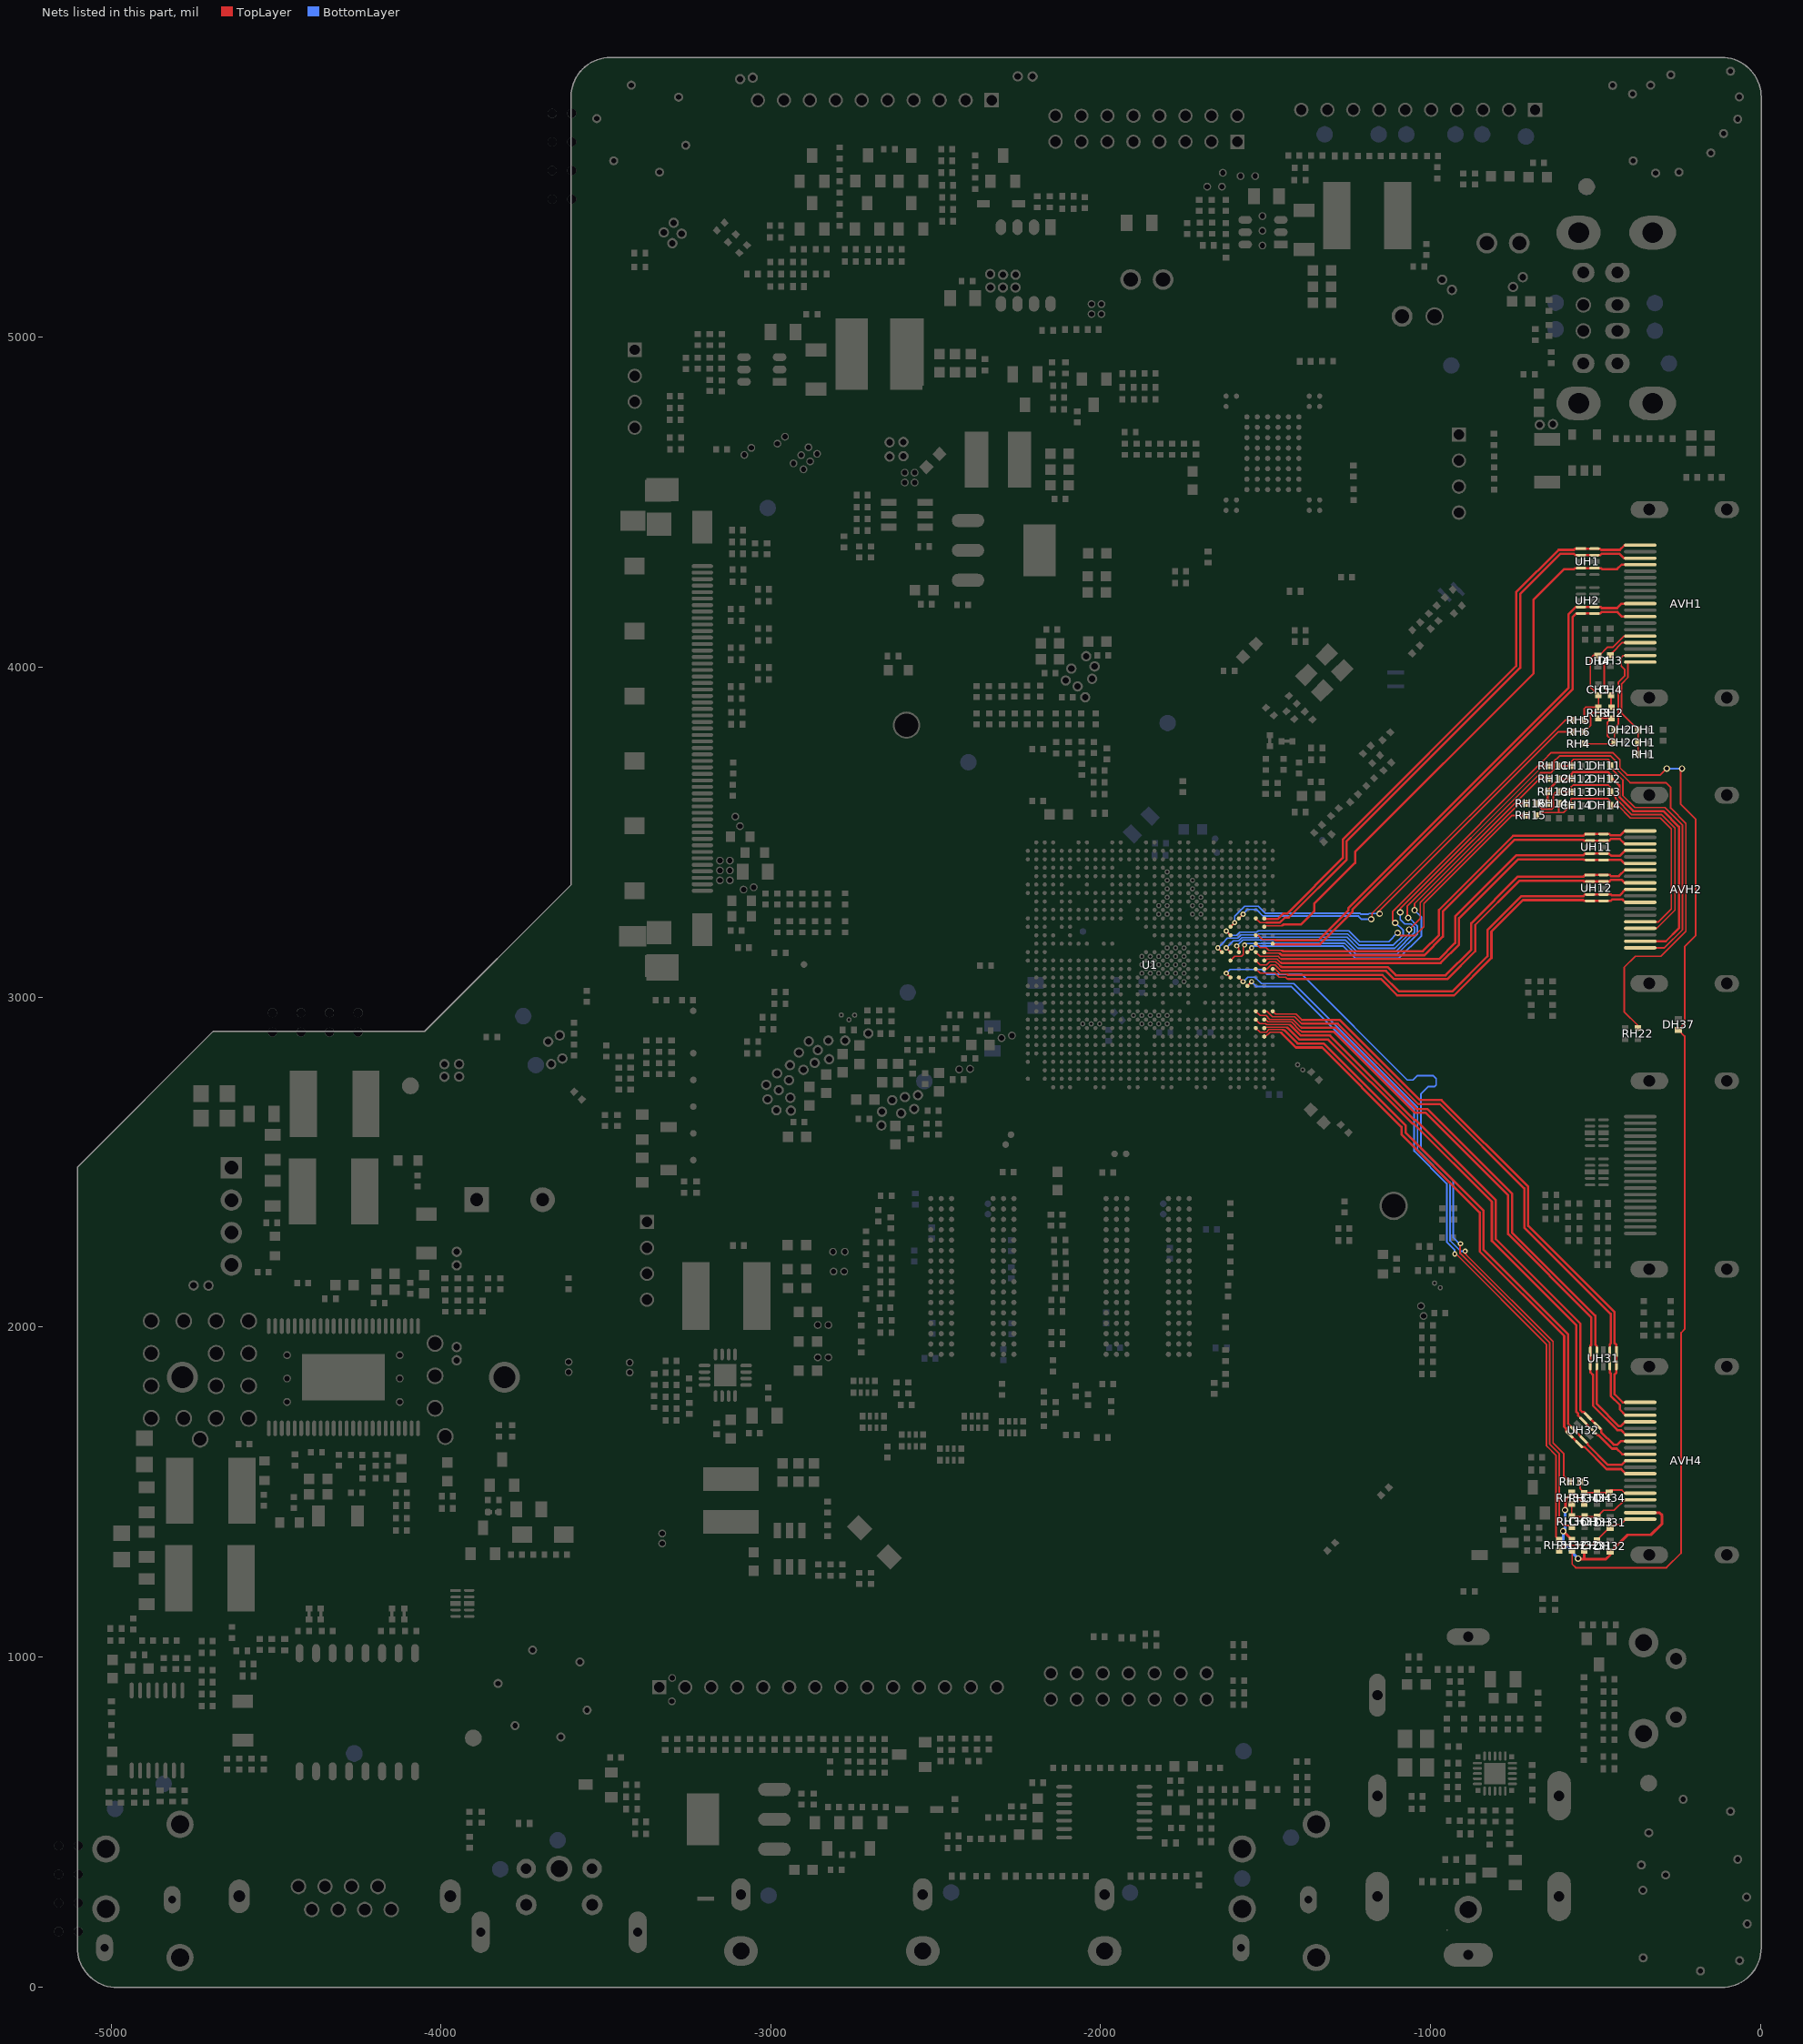
[diagram p0: the nets of this part, all layers, seen from the top]
# Altium PCB MISC86290.PcbDoc (part 22 of 31)
Units mil, origin at the board's own origin, x right, y up, seen from the top; angles counter-clockwise.
Board outline 5104.71 x 5851.49 mil, 2 copper layers (TopLayer, BottomLayer), stack 61.855 mil thick; 1026 components, 667 nets, 4280 pads, 2294 vias.

## Via types
v1: diameter 19.68, hole 11.81, TopLayer to BottomLayer, tented both sides, 1189 vias
v2: diameter 19.68/19.68 (per signal layer), hole 11.81, TopLayer to BottomLayer, tented both sides, 366 vias
v3: diameter 15.75, hole 7.87, TopLayer to BottomLayer, tented both sides, 348 vias
v4: diameter 23.62, hole 15.75, TopLayer to BottomLayer, tented both sides, 309 vias
v5: diameter 15.75/15.75 (per signal layer), hole 7.87, TopLayer to BottomLayer, tented both sides, 59 vias
v6: diameter 24/24 (per signal layer), hole 16, TopLayer to BottomLayer, tented both sides, 23 vias

## Nets (pads, with @x,y where several pads share a name; then routed paths per layer and width w, separated by ;. In a path a pad name is that pad's centre, name@x,y a point inside that pad or via, vN(x,y) a via of type N, cw(c..) or ccw(c..) an arc to the next point about the centre after c; other vN are vias at no path point) (continued)
HDMIA-RX1P: AVH1.4 U1.Y2 UH1.3 UH1.6 | length 1782.7
  TopLayer w3.94: U1.Y2@-1504.25,3213.19 -1501.3,3216.14 -1455.6,3216.14 ; -1447.61,3220.61 -1449.59,3218.63 ; -1447.39,3218.74 -1449.87,3216.26 ; -1444.95,3218.77 cw(c-1451.3,3225.12) -1449.87,3216.26 ; -1455.6,3216.14 ccw(c-1455.6,3224.64) -1449.59,3218.63 ; -1455.6,3216.14 ccw(c-1455.6,3224.64) -1449.59,3218.63 ; -1455.6,3216.14 -1451.3,3216.14 ; -1451.3,3216.14 ccw(c-1451.3,3225.12) -1449.87,3216.26 ; -1451.3,3216.14 -1449.98,3216.14 -1449.87,3216.26
  TopLayer w7: -1447.39,3218.74 -1446.01,3220.11 -1393.12,3220.11 -1351.96,3261.27 -1351.96,3283.9 -1229.06,3406.8 -1229.06,3440.01 -687.5,3981.56 -687.5,4205.09 -595.13,4297.46 -565.25,4297.46 -562.08,4300.63 UH1.3@-544.19,4300.63 UH1.6@-503.25,4300.63 -482.88,4300.63 -479.71,4297.46 -434.53,4297.46 -420.97,4311.03 AVH1.4@-365.72,4311.03
HDMIA-RX2N: AVH1.3 U1.AA3 UH1.2 UH1.7 | length 1805.1
  TopLayer w3.94: U1.AA3@-1529.84,3238.78 -1516.57,3225.51 -1497.2,3225.51
  TopLayer w7: -1497.2,3225.51 -1457.58,3225.51 -1441.98,3241.11 -1430.1,3241.11 -1254.06,3417.16 -1254.06,3472.99 -728.5,3998.55 -728.5,4222.07 -606.72,4343.86 -565.25,4343.86 -561.39,4340 UH1.2@-544.19,4340 UH1.7@-503.25,4340 -485.25,4340 -481.39,4343.86 -427.11,4343.86 -413.96,4330.71 AVH1.3@-365.72,4330.71
HDMIA-RX2P: AVH1.1 U1.AA2 UH1.1 UH1.8 | length 1775.9
  TopLayer w7: U1.AA2@-1504.25,3238.78 -1501.88,3236.41 -1463.66,3236.41 -1446.95,3253.11 -1435.07,3253.11 -1266.06,3422.13 -1266.06,3477.96 -740.5,4003.52 -740.5,4227.04 -611.69,4355.86 -565.25,4355.86 -561.42,4359.68 UH1.1@-544.19,4359.68 UH1.8@-503.25,4359.68 -486.59,4359.68 -482.76,4355.86 -426.39,4355.86 -412.17,4370.08 AVH1.1@-365.72,4370.08
HDMIA-RXCKN: AVH1.12 U1.V1 UH2.4 UH2.5 | length 1706.3
  TopLayer w3.94: U1.V1@-1478.66,3162.01 -1476.76,3160.11 -1439.67,3160.11
  TopLayer w7: U1.V1@-1476.76,3160.29 -1334.8,3160.29 -1236.85,3258.24 -1236.85,3265.34 -569.5,3932.69 -569.5,4152.01 -558.51,4163 UH2.4@-544.19,4163 -485.77,4163 -481.42,4167.35 -433.16,4167.35 -419.36,4153.55 AVH1.12@-365.72,4153.55
HDMIA-RXCKP: AVH1.10 U1.W3 UH2.3 UH2.6 | length 1762.5
  TopLayer w3.94: U1.W3@-1529.84,3187.6 -1521.97,3187.6 -1509.17,3174.8 -1477.73,3174.8 ; -1472.83,3173.01 -1473.55,3173.73 ; -1472.82,3173 ccw(c-1467.51,3178.33) -1467.51,3170.81 ; -1471.57,3172.25 ccw(c-1477.73,3166.09) -1473.55,3173.73 ; -1466.86,3172.68 ccw(c-1471.99,3167.55) -1471.77,3174.8 ; -1457.61,3172.11 -1469.08,3172.11 -1471.77,3174.8 ; -1477.73,3174.8 cw(c-1477.73,3166.09) -1473.55,3173.73 ; -1477.73,3174.8 -1474.62,3174.8 ; -1474.62,3174.8 -1471.99,3174.8 ; -1474.62,3174.8 -1473.55,3173.73 ; -1471.99,3174.8 cw(c-1471.99,3167.55) -1471.77,3174.8 ; -1471.99,3174.8 -1471.77,3174.8
  TopLayer w7: -1468.01,3172.29 -1339.77,3172.29 -1248.85,3263.21 -1248.85,3270.31 -581.5,3937.66 -581.5,4161.18 -560,4182.68 UH2.3@-544.19,4182.68 UH2.6@-503.25,4182.68 -483.93,4182.68 -480.6,4179.35 -434.53,4179.35 -420.97,4192.92 AVH1.10@-365.72,4192.92
HDMIA-SCL: AVH1.15 CH5.1 DH4.K RH3.1 RH5.1 | length 374.6
  TopLayer w5: RH5.1@-534.27,3840 -534.27,3874.46 -530,3878.73 -501.11,3878.73 ; -507.54,3878.46 RH3.1@-491,3878.46 CH5.1@-491,3915.27 -515.34,3939.61 -515.34,4027.66 -507.27,4035.73 DH4.K@-493,4035.73 -488.77,4035.73 -463.5,4061 -447.14,4061 AVH1.15@-413.65,4094.49
HDMIA-SCL_IC: RH5.2 U1.AA5 | length 1291.9
  TopLayer w3.94: U1.AA5@-1581.02,3238.78 v3(-1568.23,3251.57)
  TopLayer w5: v1@-1177.24,3238.76 -1177.24,3254.24 -591.48,3840 RH5.2@-567.73,3840
  BottomLayer w3.94: v3(-1568.23,3251.57) -1568.23,3251.77 -1554.68,3265.32 -1534.32,3265.32
  BottomLayer w5: -1534.32,3265.32 -1527.32,3265.32 -1507.67,3245.67 -1218.35,3245.67 -1208.68,3236 v1(-1180,3236)
HDMIA-SDA: AVH1.16 CH4.1 DH3.K RH2.1 RH6.1 | length 406.8
  TopLayer w5: RH6.1@-534.27,3804 -515,3823.27 -515,3857 -509.89,3862.11 -467.63,3862.11 RH2.1@-451,3878.73 -453,3880.73 CH4.1@-453,3915.27 -473.33,3935.59 -473.33,4018.14 DH3.K@-455,4036.46 ; DH3.K@-450,4044 -419.19,4074.81 AVH1.16@-364.47,4074.81
HDMIA-SDA_IC: RH6.2 U1.Y6 | length 1324.5
  TopLayer w3.94: U1.Y6@-1606.61,3213.19 v3(-1593.82,3225.98)
  TopLayer w5: v1(-1154.34,3252.61) -1158,3256.26 -1158,3259.34 -613.33,3804 RH6.2@-567.73,3804
  BottomLayer w3.94: v3(-1593.82,3225.98) -1593.82,3245.42 -1563.74,3275.5 -1522,3275.5
  BottomLayer w5: -1522,3275.5 -1501.07,3254.57 -1214.66,3254.57 -1211.69,3251.59 -1188.25,3251.59 -1186.5,3253.34 -1155.08,3253.34 v1(-1154.34,3252.61)
HDMIA_5V: AVH1.18 CH2.1 DH2.K RH2.2 RH3.2 RH4.2 | length 550.7
  TopLayer w5: RH4.2@-534.27,3768 -447,3768 CH2.1@-443,3772 CH2.1@-443.37,3772.37 ; RH3.2@-491,3845 -490.73,3845.27 RH2.2@-451,3845.27 -464,3832.27 -464,3793 CH2.1@-443.37,3772.37 ; CH2.1@-443.73,3772 CH2.1@-443.37,3772.37 ; DH2.K@-442.73,3810 -442.73,3773 CH2.1@-443.37,3772.37 ; DH2.K@-442.73,3815 -431,3826.73 -431,3953.81 -411.81,3973 -411.81,3993.73 -422.08,4004 -422.08,4029.92 -416.56,4035.44 AVH1.18@-364.47,4035.44
HDMIA_HPD: AVH1.19 CH1.1 DH1.K RH1.2 | length 336.3
  TopLayer w5: DH1.K@-376.81,3816.08 -421,3860.27 -421,3949.67 -401.81,3968.86 -401.81,4014.19 -400.25,4015.75 AVH1.19@-364.47,4015.75 ; RH1.2@-370.73,3736 DH1.K@-370.73,3810
HDMIB-DETECT: RH12.1 U1.U4 | length 1249
  TopLayer w3.94: U1.U4@-1555.43,3136.42 v3(-1542.64,3149.21)
  TopLayer w5: v1(-1048.47,3263.42) -1048.47,3283.89 -666.36,3666 RH12.1@-642.73,3666
  BottomLayer w5: v3(-1542.64,3149.21) -1537.26,3154.59 -1264.52,3154.59 -1227.96,3118.03 -1095.87,3118.03 -1027.66,3186.25 -1027.66,3242.61 v1(-1048.47,3263.42)
HDMIB-HOTPLUG: RH11.1 U1.U5 | length 1342.4
  TopLayer w3.94: v3(-1587.82,3155.21) -1581.02,3148.42 U1.U5@-1581.02,3136.42
  TopLayer w5: v1(-1092,3257) -1092,3268.64 -659.64,3701 RH11.1@-643.73,3701 ; RH11.1@-643.5,3703 RH11.1@-636.73,3703
  BottomLayer w3.94: v3(-1587.82,3155.21) -1586.32,3155.21 -1568.47,3173.06 ; -1568.28,3173.06 -1568.47,3173.06 ; -1515.81,3172.7 -1516.17,3173.06 -1568.47,3173.06
  BottomLayer w5: -1515.81,3172.7 -1257.46,3172.7 -1223.89,3139.13 -1104.61,3139.13 -1048.76,3194.99 -1048.76,3211.73 -1059.03,3222 -1078.3,3222 -1092,3235.7 v1(-1092,3257)
HDMIB-RX0N: AVH2.9 U1.R2 UH12.2 UH12.7 | length 1352.3
  TopLayer w3.94: U1.R2@-1504.25,3085.24 -1496.38,3085.24 -1483.58,3098.03 -1471.77,3098.03 -1458.88,3085.14 ; -1452.52,3078.78 -1458.87,3085.13 ccw(c-1447.31,3096.72) -1447.31,3080.35
  TopLayer w7: -1451.65,3079.35 -1135.35,3079.35 -1110.35,3054.35 -949.35,3054.35 -864.5,3139.2 -864.5,3218.96 -730.21,3353.24 -537,3353.24 -534.44,3350.68 UH12.2@-516.47,3350.68 UH12.7@-475.53,3350.68 -458.32,3350.68 -454,3355 -420,3355 -411.46,3346.46 AVH2.9@-364.47,3346.46
HDMIB-RX0P: AVH2.7 U1.T3 UH12.1 UH12.8 | length 1405.9
  TopLayer w3.94: U1.T3@-1529.84,3110.83 -1517.05,3098.03 -1497.36,3098.03 -1487.52,3107.87 -1469.8,3107.87 -1459.11,3097.19 ; -1450.29,3091.35 -1453.28,3091.35 -1456.94,3095.01 -1459.11,3097.19 ; -1459.11,3097.19 ccw(c-1448.29,3108.01) -1448.29,3092.7 cw(c-1448.29,3108.01) -1459.11,3097.19 ; -1453.27,3091.34 ccw(c-1449.68,3094.95) -1449.68,3089.86 cw(c-1449.68,3094.95) -1453.27,3091.34
  TopLayer w7: -1450.29,3091.35 -1130.38,3091.35 -1105.38,3066.35 -954.32,3066.35 -876.5,3144.17 -876.5,3223.93 -735.18,3365.24 -537,3365.24 -531.87,3370.37 UH12.1@-516.47,3370.37 UH12.8@-475.53,3370.37 -456.37,3370.37 -453,3367 -429,3367 -410.17,3385.83 AVH2.7@-364.47,3385.83
HDMIB-RX1N: AVH2.6 U1.T2 UH11.4 UH11.5 | length 1357.1
  TopLayer w3.94: U1.T2@-1504.25,3110.83 -1503.27,3109.84 -1501.3,3109.84 -1495.39,3115.75 -1465.87,3115.75 -1458.14,3108.02 ; -1453.65,3103.53 -1458.12,3108.01 ; -1450,3103.35 -1453.46,3103.35 ; -1449.52,3101.82 cw(c-1449.52,3107.66) -1453.46,3103.35 ; -1445.28,3104.87 -1450.53,3104.87 ; -1458.12,3108.01 ccw(c-1450.53,3115.63) -1450.53,3104.87 ; -1458.12,3108.01 ccw(c-1450.53,3115.63) -1450.53,3104.87 ; -1453.47,3103.36 cw(c-1449.52,3107.66) -1453.64,3103.52 -1453.47,3103.35
  TopLayer w7: -1450,3103.35 -969.65,3103.35 -913.5,3159.5 -913.5,3239.26 -734.57,3418.19 -537,3418.19 -534.44,3415.63 UH11.4@-516.47,3415.63 ; UH11.4@-516.47,3416 -475.53,3416 -423,3416 -412.51,3405.51 AVH2.6@-364.47,3405.51
HDMIB-RX1P: AVH2.4 U1.U3 UH11.3 UH11.6 | length 1372.7
  TopLayer w3.94: U1.U3@-1529.84,3136.42 -1517.05,3123.62 -1461.93,3123.62 -1457.21,3118.9 ; -1452.35,3116.89 cw(c-1452.35,3123.76) -1457.21,3118.9 ; -1450.67,3115.35 -1453.66,3115.35 ; -1450.17,3113.84 cw(c-1450.17,3118.61) -1453.55,3115.24 -1453.66,3115.35 ; -1457.21,3118.9 -1453.66,3115.35
  TopLayer w7: -1450.67,3115.35 -974.62,3115.35 -925.5,3164.47 -925.5,3244.23 -739.54,3430.19 -537,3430.19 -531.87,3435.31 UH11.3@-516.47,3435.32 UH11.6@-475.53,3435.32 -459.32,3435.32 -452,3428 -427,3428 -410.12,3444.88 AVH2.4@-364.47,3444.88
HDMIB-RX2N: AVH2.3 U1.U2 UH11.2 UH11.7 | length 1399.6
  TopLayer w3.94: U1.U2@-1504.25,3136.42 -1502.28,3136.42 -1499.33,3133.46 -1462.19,3133.46 ; -1458.78,3132.58 -1458.65,3132.45 ; -1455.4,3130.65 ccw(c-1462.19,3123.87) -1462.19,3133.46 ; -1454.82,3128.58 -1458.65,3132.45 ; -1451.16,3129.68 ccw(c-1460.29,3120.56) -1460.29,3133.46 ; -1450.68,3125.93 cw(c-1450.68,3126.2) -1450.87,3126.01 -1455.59,3130.73 ccw(c-1462.19,3124.13) -1462.19,3133.46 ; -1446.83,3127.89 cw(c-1446.83,3139.79) -1455.24,3131.37 ccw(c-1460.29,3126.33) -1460.29,3133.46 ; -1462.19,3133.46 cw(c-1462.19,3126.76) -1458.65,3132.45 ; -1462.19,3133.46 cw(c-1462.19,3126.76) -1458.65,3132.45 ; -1462.19,3133.46 -1460.29,3133.46 ; -1458.65,3132.45 cw(c-1462.19,3126.76) -1457.45,3131.5 ccw(c-1462.19,3126.76) -1458.65,3132.45
  TopLayer w7: -1454.02,3130.06 ccw(c-1447.48,3136.6) -1447.48,3127.35 ; -1450.24,3127.35 -1447.48,3127.35 ; AVH2.3@-364.47,3464.57 -411.57,3464.57 -426,3479 -454,3479 -458.32,3474.68 UH11.7@-475.53,3474.68 UH11.2@-516.47,3474.68 -534.44,3474.68 -537,3477.24 -744.81,3477.24 -962.5,3259.55 -962.5,3183.37 -1018.51,3127.35 -1447.48,3127.35
HDMIB-RX2P: AVH2.1 U1.V3 UH11.1 UH11.8 | length 1391.8
  TopLayer w3.94: U1.V3@-1529.84,3162.01 -1517.33,3149.5 -1498.63,3149.5 -1490.47,3141.34 -1454.69,3141.34 ; -1448.71,3138.86 ccw(c-1454.69,3132.88) -1448.78,3138.93 ; -1444,3139.35 ccw(c-1448.8,3134.56) -1448.8,3141.34 -1452.23,3141.34 ; -1443.73,3137.82 cw(c-1443.73,3149.83) -1448.78,3138.93 ; -1454.69,3141.34 cw(c-1454.69,3132.88) -1451.6,3140.75 ; -1454.69,3141.34 -1452.23,3141.34 ; -1452.23,3141.34 ccw(c-1443.73,3149.83) -1451.6,3140.75 ; -1451.6,3140.75 cw(c-1454.69,3132.88) -1448.78,3138.93 ; -1451.6,3140.75 ccw(c-1443.73,3149.83) -1448.78,3138.93
  TopLayer w7: -1446.8,3139.35 -1444,3139.35 -1023.49,3139.35 -974.5,3188.34 -974.5,3264.52 -749.78,3489.24 -537,3489.24 -531.87,3494.37 UH11.1@-516.47,3494.37 UH11.8@-475.53,3494.37 -458.37,3494.37 -455,3491 -424,3491 -411.06,3503.94 AVH2.1@-364.47,3503.94
HDMIB-RXCKN: AVH2.12 U1.R3 UH12.4 UH12.5 | length 1379.1
  TopLayer w3.94: U1.R3@-1529.84,3085.24 -1517.05,3072.44 -1471.77,3072.44 -1459.23,3059.9 -1438.9,3059.9 -1434.35,3055.35 ; -1435.09,3056.82 -1431.13,3056.82 ; -1431.55,3055.35 -1434.35,3055.35 ; -1430.92,3053.77 cw(c-1430.92,3058.24) -1434.08,3055.08 -1434.35,3055.35
  TopLayer w7: -1431.55,3055.35 -1150.92,3055.35 -1100.92,3005.35 -929.06,3005.35 -815.5,3118.91 -815.5,3198.66 -719.97,3294.19 -537,3294.19 -534.44,3291.63 UH12.4@-516.47,3291.63 UH12.5@-475.53,3291.63 -454.37,3291.63 -450,3296 -418,3296 -409.4,3287.4 AVH2.12@-364.47,3287.4
HDMIB-RXCKP: AVH2.10 U1.R1 UH12.3 UH12.6 | length 1338.8
  TopLayer w3.94: U1.R1@-1478.66,3085.24 -1470.79,3085.24 -1455.53,3069.98 -1439.12,3069.98 ; -1432.7,3066.6 -1435.29,3069.19 ; -1432.3,3067.16 ccw(c-1439.12,3060.34) -1435.29,3069.19 ; -1430.1,3066.6 -1430.85,3067.35 -1433.48,3069.98 ; -1429.2,3068.21 ccw(c-1433.48,3063.92) -1433.48,3069.98 ; -1439.12,3069.98 cw(c-1439.12,3060.34) -1435.29,3069.19 ; -1439.12,3069.98 -1436.08,3069.98 ; -1436.08,3069.98 -1433.48,3069.98 ; -1436.08,3069.98 -1435.29,3069.19
  TopLayer w7: -1431.55,3067.35 -1430.85,3067.35 -1145.95,3067.35 -1095.95,3017.35 -934.03,3017.35 -827.5,3123.88 -827.5,3203.63 -724.94,3306.19 -537,3306.19 -531.87,3311.31 UH12.3@-516.47,3311.32 UH12.6@-475.53,3311.32 -453.32,3311.32 -450,3308 -426.91,3308 -408.14,3326.77 AVH2.10@-364.47,3326.77
HDMIB-SCL_IC: RH15.2 U1.W6 | length 1156.4
  TopLayer w3.94: v3(-1619.41,3200.39) U1.W6@-1606.61,3187.6
  TopLayer w5: v1(-1100,3195) -1092,3187 -1047.14,3187 -1020.5,3213.64 -1020.5,3283.58 -753.08,3551 RH15.2@-712.73,3551
  BottomLayer w3.94: v3(-1619.41,3200.39) -1605.67,3186.65 -1588.13,3186.65 -1578.21,3196.57 -1527.45,3196.57 -1522.85,3201.17
  BottomLayer w5: -1522.85,3201.17 -1248.17,3201.17 -1215.03,3168.03 -1126.97,3168.03 v1(-1100,3195)
HDMIB-SDA_IC: RH16.2 U1.U6 | length 1168.5
  TopLayer w3.94: v3(-1619.41,3149.21) U1.U6@-1606.61,3136.42
  TopLayer w5: v1(-1065,3205) -1031.13,3238.87 -1031.13,3287.09 -731.22,3587 RH16.2@-712.73,3587
  BottomLayer w3.94: v3(-1619.41,3149.21) -1597.64,3170.98 -1581.63,3170.98 -1571.72,3180.89 -1520.2,3180.89
  BottomLayer w5: -1518.74,3181.6 -1518.64,3181.7 -1253.87,3181.7 -1220.2,3148.03 -1108.3,3148.03 -1065,3191.33 v1(-1065,3205)
HDMIB_5V: AVH2.18 CH12.1 DH12.K RH12.2 RH13.2 RH14.2 | length 1004.7
  TopLayer w5: AVH2.18@-364.47,3169.29 AVH2.18@-340,3169.29
  TopLayer w7: RH14.2@-644.73,3587 RH13.2@-644.73,3623 ; RH13.2@-644.73,3625.95 -610.27,3660.42 RH12.2@-610.27,3662 CH12.1@-574.73,3662.01 -574.73,3675.27 -567.33,3682.67 -502.1,3682.67 -501.11,3681.67 -461.67,3681.67 -455.27,3675.27 DH12.K@-455.27,3662 -448,3662 -427.91,3641.91 -427.91,3606.61 -385.3,3564 -294.34,3564 -247,3516.66 -247,3209 -286.71,3169.29 AVH2.18@-340,3169.29
HDMIB_HPD: AVH2.19 CH11.1 DH11.K RH11.2 | length 976.2
  TopLayer w5: RH11.2@-610.27,3701 CH11.1@-574.73,3701.01 -574.73,3713.02 -566.76,3721 -462,3721 -455.27,3714.27 DH11.K@-455.27,3701 ; DH11.K@-453.81,3699.54 -453.81,3694.81 -416.91,3657.91 -416.91,3611.16 -380.75,3575 -289.78,3575 -236,3521.22 -236,3204.44 -290.84,3149.61 AVH2.19@-364.47,3149.61
HDMIB_SCL: AVH2.15 CH14.1 DH14.K RH14.1 RH15.1 | length 867.9
  TopLayer w5: RH15.1@-679.27,3551 -670.92,3559.34 -596.4,3559.34 CH14.1@-574.73,3581.01 -574.73,3600.27 -573,3602 -463,3602 -455.27,3594.27 DH14.K@-455.27,3581 -432,3581 -394,3543 -303.04,3543 -270,3509.96 -270,3267 -308.65,3228.35 AVH2.15@-364.47,3228.35 ; -611.27,3560.08 RH14.1@-611.27,3587
HDMIB_SDA: AVH2.16 CH13.1 DH13.K RH13.1 RH16.1 | length 931.7
  TopLayer w5: RH16.1@-679.27,3587 -661.93,3569.66 -632.77,3569.66 -628,3574.42 -628,3614 -620.01,3621.99 CH13.1@-574.73,3621.99 -574.73,3636.27 -568,3643 -461.17,3643 -455.27,3637.09 DH13.K@-455.27,3622 -438.91,3605.64 -438.91,3602.05 -389.86,3553 -298.89,3553 -259,3513.11 -259,3263.86 -314.19,3208.66 AVH2.16@-364.47,3208.66
HDMIC-DETECT: DH37.K RH32.1 U1.U7 | length 4645.1
  TopLayer w3.94: v3(-1645,3149.21) U1.U7@-1632.2,3136.42
  TopLayer w5: -1114.4,3232.4 -1114.4,3260.39 -1037,3337.79 ; -1037,3338 -658.42,3716.58 ; -658.33,3716.58 -633.91,3741 -448.14,3741 -426.17,3719.03 -426.17,3695.46 -404.36,3673.64 -303.36,3673.64 v1(-284,3693) ; RH32.1@-571,1321.27 -571,1281 -560.25,1270.25 -284.75,1270.25 -240.5,1314.5 -240.5,1982.5 -229.66,1993.34 -229.66,2881.52 DH37.K@-248.64,2900.5 -229.66,2919.48 -229.66,3153.2 -196,3186.86 -196,3539.25 -242,3585.25 v1@-242,3689
  BottomLayer w3.94: v3(-1645,3149.21) -1631.22,3162.99 -1615.4,3178.81 -1584.88,3178.81 -1574.96,3188.73 -1523.45,3188.73 -1520.58,3191.6
  BottomLayer w5: -1520.58,3191.6 -1251.19,3191.6 -1217.62,3158.03 -1112.44,3158.03 -1082.66,3187.82 -1082.66,3202.18 v1@-1105.47,3225 ; v1(-284,3693) v1(-238,3693)
  other v1: -1107,3225
HDMIC-HOTPLUG: RH31.1 U1.N4 | length 2159.6
  TopLayer w3.94: U1.N4@-1555.43,3034.06 v3(-1542.64,3046.85)
  TopLayer w5: v3(-926.47,2221.66) v3@-924.76,2219.89 ; v3@-923.02,2221.63 -648.88,1947.49 -648.88,1639.95 -645.95,1637.02 -619.84,1610.92 -619.84,1364.57 RH31.1@-610,1354.73
  BottomLayer w5: v3(-1542.64,3046.85) -1527.6,3031.81 -1421.81,3031.81 -1049.5,2659.5 -1049.5,2533.3 -951,2434.8 -951,2257.64 -927,2233.64 -927,2222.2 v3(-926.47,2221.66)
HDMIC-RX0N: AVH4.9 U1.H2 UH32.2 UH32.7 | length 1917.7
  TopLayer w3.94: U1.H2@-1504.25,2906.1 -1501.3,2909.06 -1441.45,2909.06 ; -1434.14,2907.56 -1435.63,2909.06 -1441.45,2909.06 ; -1441.45,2909.06 cw(c-1441.45,2900.26) -1435.23,2906.48 ccw(c-1441.45,2900.26) -1441.45,2909.06
  TopLayer w7: -1434.14,2907.56 -1397.97,2871.4 -1309.93,2871.4 -1054.53,2616 -1050.65,2616 -814.09,2379.44 -814.09,2261.19 -557.88,2004.98 -557.88,1742.91 -552.49,1737.51 -552.49,1731.16 UH32.2@-537.11,1715.79 UH32.7@-508.16,1686.84 -493.84,1672.51 -491.49,1672.51 -450.14,1631.17 -436.14,1631.17 -419.14,1614.17 AVH4.9@-364.47,1614.17
HDMIC-RX0P: AVH4.7 U1.J3 UH32.1 UH32.8 | length 1937
  TopLayer w3.94: U1.J3@-1529.84,2931.69 -1517.62,2919.47 -1500.41,2919.47 -1497.87,2916.93 -1431.87,2916.93 ; -1426.58,2914.74 ccw(c-1431.87,2909.44) -1431.87,2916.93 ; -1425.04,2915.43 -1426.53,2916.93 -1431.87,2916.93
  TopLayer w7: -1425.04,2915.43 -1393,2883.4 -1304.96,2883.4 -1049.56,2628 -1045.68,2628 -802.09,2384.41 -802.09,2266.16 -545.88,2009.95 -545.88,1747.88 -540,1742 -535.48,1742 UH32.1@-523.19,1729.71 -483,1689.52 -483,1681 -445.17,1643.17 -434,1643.17 -423.63,1653.54 AVH4.7@-364.47,1653.54
HDMIC-RX1N: AVH4.6 U1.J2 UH31.4 UH31.5 | length 1899.8
  TopLayer w3.94: U1.J2@-1504.25,2931.69 -1499.86,2931.69 -1492.97,2924.8 -1421.16,2924.8 -1396.11,2899.75 ; -1391.76,2895.4 -1396.11,2899.75 ; -1396.11,2899.75 ccw(c-1389.15,2906.71) -1389.15,2896.87 cw(c-1389.15,2906.71) -1396.11,2899.75
  TopLayer w7: -1389.59,2895.4 -1293.93,2895.4 -1047.53,2649 -1014.35,2649 -765.09,2399.74 -765.09,2281.49 -513,2029.4 -513,1945 -515,1943 -515,1926.05 UH31.4@-515.63,1925.42 UH31.5@-515.63,1884.48 -515.63,1862.63 -507.94,1854.94 -507.94,1761.45 -433.79,1687.3 -422.21,1687.3 -408.14,1673.23 AVH4.6@-364.47,1673.23
HDMIC-RX1P: AVH4.4 U1.K3 UH31.3 UH31.6 | length 1922
  TopLayer w3.94: U1.K3@-1529.84,2957.28 -1517.05,2944.49 -1499.33,2944.49 -1487.52,2932.68 -1417.95,2932.68 -1396.66,2911.38 ; -1390.56,2908.86 cw(c-1390.56,2917.48) -1396.66,2911.38 ; -1390.51,2907.4 -1392.67,2907.4 -1396.66,2911.38
  TopLayer w7: -1390.51,2907.4 -1288.96,2907.4 -1042.56,2661 -1009.38,2661 -753.09,2404.71 -753.09,2286.46 -501,2034.37 -501,1947 -495.94,1941.94 UH31.3@-495.94,1925.42 UH31.6@-495.94,1884.48 -495.94,1766.42 -428.82,1699.3 -424,1699.3 -410.7,1712.6 AVH4.4@-364.47,1712.6
HDMIC-RX2N: AVH4.3 U1.K2 UH31.2 UH31.7 | length 1889.5
  TopLayer w3.94: U1.K2@-1504.25,2957.28 -1495.87,2957.28 -1479.14,2940.55 -1411.73,2940.55 -1394.38,2923.19 ; -1390.16,2918.97 ccw(c-1387.56,2921.58) -1387.56,2917.9 ; -1390.16,2918.98 -1394.38,2923.19 ; -1383.97,2920.91 -1388.86,2920.91 ; -1394.38,2923.19 ccw(c-1388.86,2928.71) -1388.86,2920.91 ; -1394.38,2923.19 ccw(c-1388.86,2928.71) -1388.86,2920.91
  TopLayer w7: -1387.65,2919.4 -1281.02,2919.4 -1037.28,2675.66 -971.71,2675.66 -716.09,2420.04 -716.09,2301.79 -454,2039.69 -454,1950 -456.57,1947.43 UH31.2@-456.57,1925.42 UH31.7@-456.57,1884.48 -456.57,1861.57 -454,1859 -454,1791.03 -426,1763.03 -426,1750.14 -408.14,1732.28 AVH4.3@-364.47,1732.28
HDMIC-RX2P: AVH4.1 U1.K1 UH31.1 UH31.8 | length 1827.8
  TopLayer w3.94: U1.K1@-1478.66,2957.28 -1469.8,2948.43 -1408.11,2948.43 -1393.98,2934.29 ; -1390.54,2932.87 cw(c-1390.54,2937.73) -1393.97,2934.29 -1390.21,2930.53
  TopLayer w7: -1389.33,2931.4 -1276.05,2931.4 -1032.31,2687.66 -966.74,2687.66 -704.09,2425.01 -704.09,2306.76 -442,2044.67 -442,1951 -436.89,1945.89 UH31.1@-436.89,1925.42 UH31.8@-436.89,1884.48 -436.89,1861.11 -442,1856 -442,1796 -417.65,1771.65 AVH4.1@-364.47,1771.65
HDMIC-RXCKN: AVH4.12 U1.G2 UH32.4 UH32.5 | length 1958.4
  TopLayer w3.94: U1.G2@-1504.25,2880.51 -1499.47,2880.51 -1486.67,2893.31 -1458.83,2893.31 ; -1452.33,2891.81 -1453.82,2893.31 -1458.83,2893.31 ; -1458.83,2893.31 cw(c-1458.83,2886.3) -1453.87,2891.25 ccw(c-1458.83,2886.3) -1458.83,2893.31
  TopLayer w7: -1452.33,2891.81 -1407.9,2847.39 -1328.86,2847.39 -1088,2606.53 -1088,2584.06 -851.09,2347.15 -851.09,2228.9 -594.88,1972.68 -594.88,1697.88 -589,1692 -589,1684.16 UH32.4@-578.87,1674.03 UH32.5@-549.92,1645.08 -541.34,1636.5 -533.5,1636.5 -466.16,1569.16 -422.18,1569.16 -408.14,1555.12 AVH4.12@-364.47,1555.12
HDMIC-RXCKP: AVH4.10 U1.H3 UH32.3 UH32.6 | length 1984.6
  TopLayer w3.94: U1.H3@-1529.84,2906.1 -1517.05,2893.31 -1497.76,2893.31 -1489.88,2901.18 -1450.8,2901.18 ; -1443.23,2899.69 -1444.73,2901.18 -1450.8,2901.18 ; -1450.8,2901.18 cw(c-1450.8,2891.19) -1443.73,2898.25 ccw(c-1450.8,2891.19) -1450.8,2901.18
  TopLayer w7: -1443.23,2899.69 -1402.93,2859.39 -1323.89,2859.39 -1076,2611.5 -1076,2589.03 -839.09,2352.12 -839.09,2233.87 -582.88,1977.65 -582.88,1705.88 UH32.3@-564.95,1687.95 UH32.6@-536,1659 -523.92,1646.92 -523.92,1643.89 -462.03,1582 -420.63,1582 -408.14,1594.49 AVH4.10@-364.47,1594.49
HDMIC-SCL_IC: RH35.2 U1.P5 | length 2056.7
  TopLayer w3.94: U1.P5@-1581.02,3059.65 v3(-1568.23,3046.85)
  TopLayer w5: v3(-895,2230) -895.5,2230 -899.3,2226.2 -881.59,2208.48 ; -883.55,2210.45 -628.88,1955.77 -628.88,1648.24 -596.09,1615.45 -596.09,1547.36 RH35.2@-579.73,1531
  BottomLayer w3.94: v3(-1568.23,3046.85) -1554.45,3060.63 -1532.32,3060.63 -1530.08,3058.39
  BottomLayer w5: -1530.08,3058.39 -1512.96,3041.27 -1414.27,3041.27 -1039.5,2666.5 -1039.5,2537.44 -941,2438.94 -941,2261.78 -909.22,2230 v3(-895,2230)
HDMIC-SDA_IC: RH36.2 U1.P6 | length 2401.5
  TopLayer w3.94: v3(-1619.41,3072.44) U1.P6@-1606.61,3059.65
  TopLayer w5: v3(-909.5,2252.5) -910.37,2251.63 -910.37,2223.13 -638.88,1951.63 -638.88,1644.09 -609.84,1615.06 -609.84,1411.84 -596.34,1398.34 -576.07,1398.34 RH36.2@-571,1393.27
  BottomLayer w3.94: v3(-1619.41,3072.44) -1607.56,3084.29 -1510.98,3084.29 ; -1510.94,3084.25 -1506.86,3080.17
  BottomLayer w5: -1506.86,3080.17 -1496.34,3069.65 -1391.51,3069.65 -1070.51,2748.66 -1052.95,2748.66 -1039.37,2762.24 -992.77,2762.24 -983.26,2752.73 -983.26,2733.85 -988.68,2728.43 -1007.38,2728.43 -1029.5,2706.31 -1029.5,2541.58 -931,2443.08 -931,2271 -912.5,2252.5 v3(-909.5,2252.5)
HDMIC_5V: AVH4.18 CH32.1 DH32.K RH32.2 RH33.2 RH34.2 | length 746.6
  TopLayer w8: v2(-598,1381) -571.73,1354.73 RH32.2@-571,1354.73 ; v1(-592.5,1445) -591.43,1445 -590.84,1445.59 -590.84,1476.85 -572,1495.7 RH33.2@-572,1497.73 -568.46,1497.73 RH34.2@-534,1463.27 ; v1(-553,1298) -551,1296 -468.59,1296 -456,1308.59 DH32.K@-456,1319.27 -453.09,1319.27 -402.35,1370 -332,1370 -298,1404 -298,1429 -306.01,1437.01 AVH4.18@-364.47,1437.01 ; -534,1297 CH32.1@-534,1321.27
  BottomLayer w8: v1(-592.5,1445) -592.5,1388.5 -599,1382 v2(-598,1381) -598,1347 -579.02,1328.02 -579.02,1324.02 v1(-553,1298)
HDMIC_HPD: AVH4.19 CH31.1 DH31.K RH31.2 | length 282.6
  TopLayer w5: RH31.2@-610,1321.27 -592.89,1338.37 -510.63,1338.37 CH31.1@-496,1353 DH31.K@-458.73,1390.27 ; DH31.K@-456,1390.27 -446,1400.27 -424.73,1400.27 -409,1416 AVH4.19@-365.8,1416
  TopLayer w8: AVH4.19@-365.8,1416 AVH4.19@-364.47,1417.32
HDMIC_SCL: AVH4.15 CH34.1 DH34.K RH34.1 RH35.1 | length 214.1
  TopLayer w5: RH35.1@-546.27,1531 -546.27,1509 RH34.1@-534,1496.73 -533,1497.73 CH34.1@-496,1497.73 DH34.K@-458,1497.73 DH34.K@-456.02,1495.75 ; DH34.K@-456.02,1505.75 -420,1505.75 -410.31,1496.06 AVH4.15@-364.47,1496.06
HDMIC_SDA: AVH4.16 CH33.1 DH33.K RH33.1 RH36.1 | length 268
  TopLayer w5: RH33.1@-572,1464.27 -572,1427.73 RH36.1@-571,1426.73 -569,1424.73 DH33.K@-495,1424.73 -475.51,1444.22 -443.78,1444.22 -410,1478 -366.09,1478 AVH4.16@-364.47,1476.38
HDMID-DETECT: RH22.1 U1.T6 | length 2673.6
  TopLayer w3.94: U1.T6@-1606.61,3110.83 -1593.19,3124.25 -1573.45,3124.25 -1567.9,3129.8 -1567.9,3154.2 v3@-1564,3158.1
  TopLayer w5: v1@-1071,3240.3 -1071,3275.5 -666.5,3680 -635.43,3680 -626.73,3688.69 -626.73,3713.84 -609.58,3731 -454,3731 -436.17,3713.17 -436.17,3691.31 -394.86,3650 -287,3650 -272,3635 -272,3572.82 -226,3526.82 -226,3199.28 -301.28,3124 -379,3124 -413,3090 -413,2956 -372,2915 RH22.1@-372,2905.73
  BottomLayer w3.94: v3@-1560.64,3162.96 -1513.72,3162.96
  BottomLayer w5: -1513.18,3163.5 -1260.85,3163.5 -1227.58,3130.23 -1100.93,3130.23 -1039.86,3191.3 -1039.86,3215.41 v1@-1064.74,3240.3
  other v1: -1067.7,3240.3
  other v3: -1563.9,3158.1